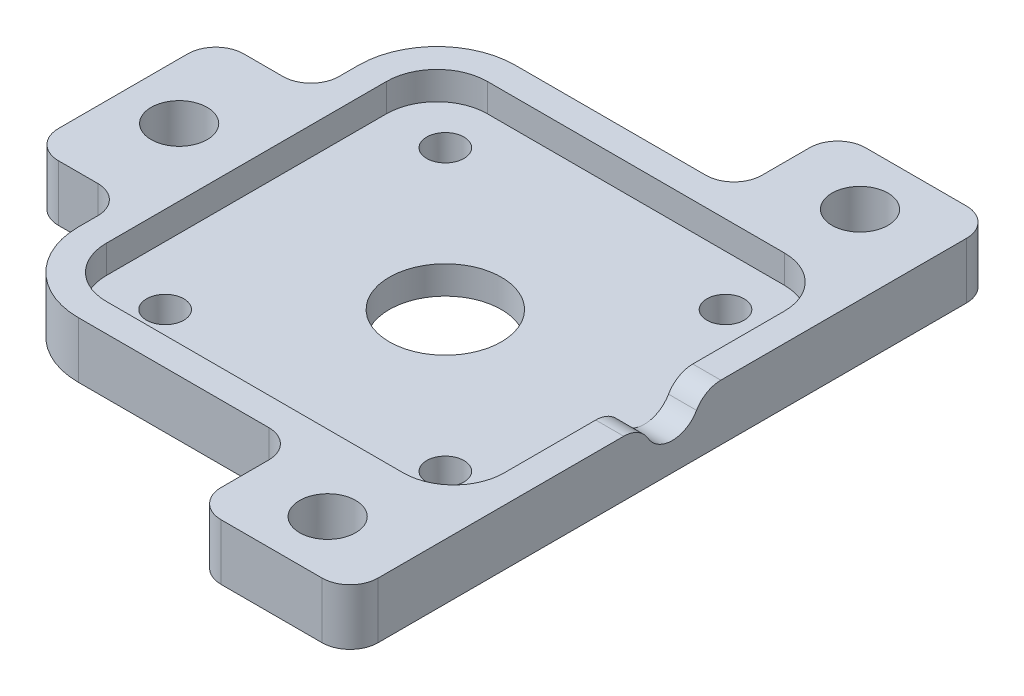
SolidWorks part; units mm, degrees
ref_plane "Front Plane" through (0, 0, 0) normal (0, 0, 1) x (1, 0, 0)
ref_plane "Top Plane" through (0, 0, 0) normal (0, 1, 0) x (1, 0, 0)
ref_plane "Right Plane" through (0, 0, 0) normal (1, 0, 0) x (0, 0, -1)
sketch "Sketch1" plane through (0, 0, 0) normal (0, 1, 0) x (1, 0, 0)
  line L0 (-40.5, 39) -> (40.5, 39)
  line L1 (-35.5, 34) -> (35.5, 34)
  line L2 (-35.5, 34) -> (-35.5, -34)
  line L3 (-35.5, -34) -> (35.5, -34)
  line L4 (35.5, 34) -> (35.5, -34)
  line L5 (-35.5, 34) -> (35.5, -34) construction
  line L6 (-35.5, -34) -> (35.5, 34) construction
  line L7 (40.5, 39) -> (40.5, -39)
  line L8 (-40.5, -39) -> (40.5, -39)
  line L9 (-40.5, 39) -> (-40.5, -39)
  point P0 (0, 0)
  dimension "D1" = 71
  dimension "D2" = 68
  dimension "D3" = 5
extrude "Boss-Extrude1" add sketch "Sketch1" along normal blind 5
sketch "Sketch2" plane through (0, 0, 0) normal (0, -1, 0) x (1, 0, 0)
  line L5 (40.5, -39) -> (-40.5, -39)
  line L6 (40.5, -39) -> (40.5, 39)
  line L7 (40.5, 39) -> (-40.5, 39)
  line L8 (-40.5, -39) -> (-40.5, 39)
  line L9 (40.5, -39) -> (-40.5, 39) construction
  line L10 (40.5, 39) -> (-40.5, -39) construction
  point P0 (0, 0)
extrude "Boss-Extrude2" add sketch "Sketch2" along normal blind 5
sketch "Sketch3" plane through (0, -5, 0) normal (0, -1, 0) x (1, 0, 0)
  line L0 (0, 0) -> (-53.4262, 0) construction
  line L1 (0, 0) -> (0, 49.2788) construction
  line L2 (-42.5, 16.526) -> (-57.5, 16.526)
  line L3 (-42.5, 42.5) -> (-42.5, -42.5) construction
  line L4 (-57.5, 16.526) -> (-57.5, 1.526)
  line L6 (40.5, 57.5) -> (12.5, 57.5)
  line L7 (12.5, 57.5) -> (12.5, 42.5)
  line L8 (42.5, 42.5) -> (-42.5, 42.5) construction
  line L14 (-57.5, -16.526) -> (-57.5, -1.526)
  line L15 (-43.1294, -16.526) -> (-57.5, -16.526)
  line L16 (-57.5, 1.526) -> (-57.5, -1.526)
  line L18 (-42.5, 16.526) -> (-40.5, 16.526)
  line L19 (40.5, 39) -> (40.5, 57.5)
  line L20 (-40.5, 39) -> (-40.5, -39) construction
  line L21 (-40.5, 16.526) -> (-40.5, -16.526)
  line L22 (-40.5, -16.526) -> (-43.1294, -16.526)
  line L23 (12.5, 42.5) -> (12.5, 39)
  line L24 (40.5, 39) -> (-40.5, 39) construction
  line L25 (12.5, 39) -> (40.5, 39)
  line L26 (12.5, -39) -> (40.5, -39)
  line L27 (12.5, -42.5) -> (12.5, -39)
  line L28 (40.5, -39) -> (40.5, -57.5)
  line L29 (12.5, -57.5) -> (12.5, -42.5)
  line L30 (40.5, -57.5) -> (12.5, -57.5)
  dimension "D1" = 15
  dimension "D2" = 15
extrude "Boss-Extrude3" add sketch "Sketch3" against normal blind 10
fillet "Fillet1" radius 9 4 edges at (-35.5, 2.5, 34) (35.5, 2.5, 34) (35.5, 2.5, -34) (-35.5, 2.5, -34)
fillet "Fillet2" radius 14 2 edges at (-40.5, 0, 39) (-40.5, 0, -39)
fillet "Fillet4" radius 5 10 edges at (40.5, 0, 57.5) (12.5, 0, 57.5) (12.5, 0, 39) (-40.5, 0, 16.526) (-57.5, 0, 16.526) (12.5, 0, -39) (-57.5, 0, -16.526) (40.5, 0, -57.5) (12.5, 0, -57.5) (-40.5, 0, -16.526)
sketch "Sketch4" plane through (0, 0, 0) normal (0, 1, 0) x (1, 0, 0)
  circle A0 centre (0, 0) radius 10
  dimension "D1" = 20
extrude "Cut-Extrude1" cut sketch "Sketch4" against normal blind 5
sketch "Sketch5" plane through (0, 5, 0) normal (0, 1, 0) x (1, 0, 0)
  line L0 (-57.5, 0) -> (-35.5, 0) construction
  line L1 (-57.5, -11.526) -> (-57.5, 11.526) construction
  line L2 (-35.5, 25) -> (-35.5, -25) construction
  line L3 (26.5, 57.5) -> (26.5, 39.7046) construction
  line L4 (17.5, 57.5) -> (35.5, 57.5) construction
  line L5 (26.5, -57.5) -> (26.5, -37.5) construction
  line L6 (35.5, -57.5) -> (17.5, -57.5) construction
  circle A0 centre (-47.5, 0) radius 5
  circle A1 centre (26.5, 47.5) radius 5
  circle A2 centre (26.5, -47.5) radius 5
  dimension "D4" = 10
  dimension "D5" = 10
  dimension "D6" = 10
  dimension "D1" = 10
  dimension "D2" = 10
  dimension "D3" = 10
extrude "Cut-Extrude2" cut sketch "Sketch5" against normal blind 24 contours A1 | A2 | A0
sketch "Sketch6" plane through (40.5, 0, 0) normal (1, 0, 0) x (0, 0, -1)
  line L0 (-52.5, 5) -> (52.5, 5) construction
  circle A0 centre (0, 5) radius 5
extrude "Cut-Extrude3" cut sketch "Sketch6" against normal blind 5
fillet "Fillet5" radius 5 2 edges at (38, 5, 5) (38, 5, -5)
sketch "Sketch7" plane through (0, 5, 0) normal (0, 1, 0) x (1, 0, 0)
  circle A0 centre (25, 25) radius 3.3235
  circle A1 centre (-25, 25) radius 3.3235
  circle A2 centre (-25, -25) radius 3.3235
  circle A3 centre (25, -25) radius 3.3235
extrude "Cut-Extrude4" cut sketch "Sketch7" against normal blind 10
